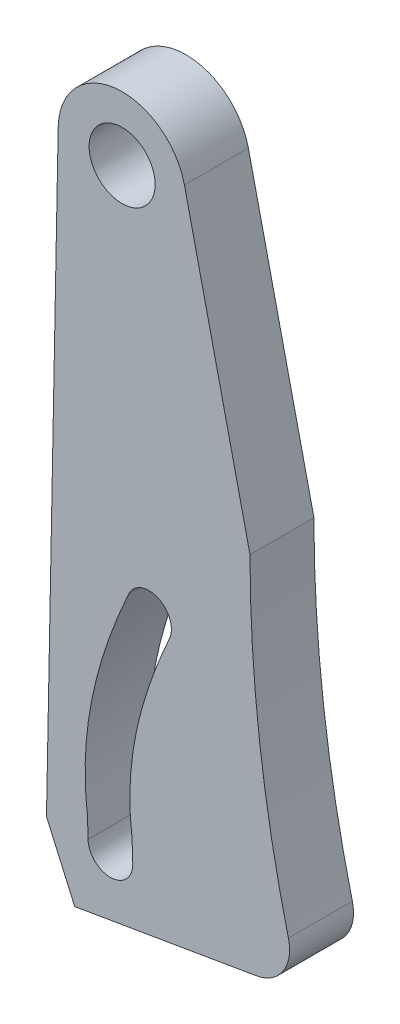
SolidWorks part; units mm, degrees
material "Thornel Mat VMA"
ref_plane "前视基准面" through (0, 0, 0) normal (0, 0, 1) x (1, 0, 0)
ref_plane "上视基准面" through (0, 0, 0) normal (0, 1, 0) x (1, 0, 0)
ref_plane "右视基准面" through (0, 0, 0) normal (1, 0, 0) x (0, 0, -1)
other "Configuration Table"
sketch "草图1"
  line L0 (3.8162, 0.7114) -> (0.7411, 14.1914)
  line L1 (-2.1838, 13.5241) -> (3.8162, -14.4209) construction
  line L2 (-2.1838, 13.5241) -> (-2.7337, -14.6313) construction
  line L3 (-2.1838, 13.5241) -> (-2.7471, -14.0898) construction
  line L4 (-2.1838, 13.5241) -> (-2.7731, -13.5291) construction
  line L5 (-2.1838, 13.5241) -> (-2.8303, -12.9865) construction
  line L6 (-2.1838, 13.5241) -> (-2.8637, -12.4261) construction
  line L7 (-2.1838, 13.5241) -> (-2.8697, -11.8608) construction
  line L8 (-2.1838, 13.5241) -> (-2.8529, -11.291) construction
  line L9 (-2.1838, 13.5241) -> (-2.8123, -10.717) construction
  line L10 (-2.1838, 13.5241) -> (-2.7482, -10.1392) construction
  line L11 (-2.1838, 13.5241) -> (-2.661, -9.5577) construction
  line L12 (-2.1838, 13.5241) -> (-2.5512, -8.9728) construction
  line L13 (-2.1838, 13.5241) -> (-2.4192, -8.3846) construction
  line L14 (-2.1838, 13.5241) -> (-2.2655, -7.793) construction
  line L15 (-2.1838, 13.5241) -> (-2.0907, -7.1983) construction
  line L16 (-2.1838, 13.5241) -> (-1.8954, -6.6001) construction
  line L17 (-2.1838, 13.5241) -> (-1.6801, -5.9985) construction
  line L18 (-2.1838, 13.5241) -> (-1.4455, -5.3931) construction
  line L19 (-2.1838, 13.5241) -> (-1.1925, -4.7837) construction
  line L20 (-2.1838, 13.5241) -> (-0.9217, -4.1699) construction
  line L21 (-0.9217, -4.1699) -> (-1.1925, -4.7837) construction
  line L22 (-1.1925, -4.7837) -> (-1.4455, -5.3931) construction
  line L23 (0.0301, -4.6131) -> (-0.9217, -4.1699) construction
  line L24 (-2.1622, -4.381) -> (-0.2228, -5.1864) construction
  line L25 (-1.4455, -5.3931) -> (-1.6801, -5.9985) construction
  line L26 (-1.6801, -5.9985) -> (-1.8954, -6.6001) construction
  line L27 (-2.4246, -5.0138) -> (-0.4664, -5.7724) construction
  line L28 (-2.6687, -5.6447) -> (-0.6915, -6.3522) construction
  line L29 (-1.8954, -6.6001) -> (-2.0907, -7.1983) construction
  line L30 (-2.8935, -6.2741) -> (-0.8972, -6.9261) construction
  line L31 (-2.0907, -7.1983) -> (-2.2655, -7.793) construction
  line L32 (-3.0981, -6.9022) -> (-1.0833, -7.4943) construction
  line L33 (-2.2655, -7.793) -> (-2.4192, -8.3846) construction
  line L34 (-3.2818, -7.529) -> (-1.2492, -8.057) construction
  line L35 (-3.4437, -8.1547) -> (-1.3946, -8.6144) construction
  line L36 (-2.4192, -8.3846) -> (-2.5512, -8.9728) construction
  line L37 (-2.5512, -8.9728) -> (-2.661, -9.5577) construction
  line L38 (-3.5831, -8.7791) -> (-1.5192, -9.1666) construction
  line L39 (-2.661, -9.5577) -> (-2.7482, -10.1392) construction
  line L40 (-3.6994, -9.402) -> (-1.6226, -9.7134) construction
  line L41 (-2.7482, -10.1392) -> (-2.8123, -10.717) construction
  line L42 (-3.7917, -10.0234) -> (-1.7046, -10.255) construction
  line L43 (-2.7482, -10.1392) -> (-2.8123, -10.717) construction
  line L44 (-2.8123, -10.717) -> (-2.8529, -11.291) construction
  line L45 (-2.8529, -11.291) -> (-2.8697, -11.8608) construction
  line L46 (-2.8697, -11.8608) -> (-2.8637, -12.4261) construction
  line L47 (-2.8637, -12.4261) -> (-2.8303, -12.9865) construction
  line L48 (-2.8303, -12.9865) -> (-2.7731, -13.5291) construction
  line L49 (-3.8597, -10.6429) -> (-1.7649, -10.7912) construction
  line L50 (-3.9025, -11.2601) -> (-1.8034, -11.3219) construction
  line L51 (-3.9196, -11.8719) -> (-1.8198, -11.8497) construction
  line L52 (-3.9119, -12.4886) -> (-1.8156, -12.3636) construction
  line L53 (-2.8303, -12.9865) -> (-2.7731, -13.5291) construction
  line L54 (-3.8745, -13.0967) -> (-1.7861, -12.8764) construction
  line L55 (-2.7731, -13.5291) -> (-2.7471, -14.0898) construction
  line L56 (-3.8219, -13.5777) -> (-1.7242, -13.4806) construction
  line L57 (-3.7968, -14.1158) -> (-1.6974, -14.0638) construction
  line L58 (-2.7471, -14.0898) -> (-2.7337, -14.6313) construction
  line L59 (-2.7337, -14.6313) -> (-1.684, -14.6053) construction
  line L60 (-2.7337, -14.6313) -> (-3.7834, -14.6573) construction
  line L61 (-2.7337, -14.6313) -> (-4.4081, -17.7048) construction
  line L62 (-2.7337, -14.6313) -> (-5.7328, -14.7056) construction
  line L63 (-4.4081, -17.7048) -> (4.1278, -16.2526)
  line L64 (-5.7328, -14.7056) -> (-4.4081, -17.7048)
  line L65 (-5.7328, -14.7056) -> (-5.1832, 13.5824)
  line L66 (-0.9217, -4.1699) -> (-1.8824, -3.7461) construction
  circle A0 centre (-2.1838, 13.5241) radius 1.55
  arc A1 (3.8162, 0.7114) -> (5.619, -13.9714) centre (64.5084, 0.7114) ccw
  arc A2 (0.7411, 14.1914) -> (-5.1832, 13.5824) centre (-2.1838, 13.5241) ccw
  arc A3 (4.1278, -16.2526) -> (5.619, -13.9714) centre (3.8162, -14.4209) ccw
  arc A4 (-3.7834, -14.6573) -> (-1.684, -14.6053) centre (-2.7337, -14.6313) ccw
  arc A12 (0.0301, -4.6131) -> (-1.8824, -3.7461) centre (-0.9217, -4.1699) ccw
  spline S0 degree 3 poles (-3.7834, -14.6573) (-3.7993, -14.2982) (-3.7863, -13.7741) (-3.8865, -13.0558) (-3.9159, -12.4861) (-3.9238, -11.8735) (-3.9066, -11.2577) (-3.8491, -10.4322) (-3.741, -9.6037) (-3.5864, -8.7763) (-3.4467, -8.1517) (-3.2845, -7.5259) (-3.1005, -6.8989) (-2.8956, -6.2707) (-2.6705, -5.6411) (-2.3426, -4.7944) (-2.072, -4.1648) (-1.8824, -3.7461) knots 0 0 0 0 0.09621 0.139298 0.193554 0.248477 0.302979 0.358078 0.469497 0.525932 0.582904 0.640455 0.698625 0.757451 0.81697 0.877215 1 1 1 1
  spline S1 degree 3 poles (-1.684, -14.6053) (-1.6984, -14.2309) (-1.6906, -13.6511) (-1.7908, -12.9082) (-1.8196, -12.3636) (-1.8228, -11.845) (-1.8071, -11.3204) (-1.7682, -10.7884) (-1.7076, -10.2519) (-1.6254, -9.71) (-1.486, -8.9741) (-1.3512, -8.4238) (-1.2492, -8.057) knots 0 0 0 0 0.170355 0.262297 0.340044 0.417824 0.497759 0.578301 0.659977 0.742887 0.827132 1 1 1 1
  spline S2 degree 3 poles (0.0301, -4.6131) (-0.1433, -4.9961) (-0.3915, -5.5728) (-0.6925, -6.3475) (-0.9647, -7.1056) (-1.1434, -7.6766) (-1.2492, -8.057) knots 0 0 0 0 0.34298 0.512099 0.67788 1 1 1 1
other "对齐组1" parameters "D1"=3.1, "D2"=3.1, "D3"=6, "D4"=3.1, "D6"=60.6922, "D9"=3.716, "D29"=1.6132, "D31"=2, "D33"=2, "D35"=2, "D37"=2, "D39"=2, "D41"=2, "D43"=2, "D45"=2, "D47"=2, "D49"=2, "D52"=10.768, "D59"=2.05, "D71"=2, "D84"=2, "D85"=2.1, "D5"=13.8263, "D7"=3.8162, "D8"=5.619, "D10"=3.8162, "D11"=26.7925, "D12"=26.7823, "D13"=26.7925, "D14"=25.5532, "D15"=26.2854, "D16"=27.0533, "D17"=21.6117, "D18"=19.2403, "D19"=20.3681, "D20"=20.7218, "D21"=22.5274, "D22"=24.4408, "D23"=20.4903, "D24"=21.1433, "D25"=20.0275, "D26"=17.4108, "D27"=21.8201, "D28"=20.5543, "D30"=27.945, "D32"=16.1585, "D34"=21.91, "D36"=21.3173, "D38"=18.0374, "D40"=15.8792, "D42"=15.2189, "D44"=14.1906, "D46"=18.3346, "D48"=17.739, "D50"=1, "D51"=0.6492, "D53"=1, "D54"=1, "D55"=0.8492, "D56"=0.8492, "D57"=0.6292, "D58"=1.1033, "D60"=1.1166, "D61"=0.6111, "D62"=1.142, "D63"=1.3101, "D64"=0.6029, "D65"=0.5951, "D66"=1.0637, "D67"=0.588, "D68"=1.2009, "D69"=0.5814, "D70"=1.0157, "D72"=0.5754, "D73"=0.402, "D74"=0.402, "D75"=1.1507, "D76"=1.1506, "D77"=0.9199, "D78"=0.9199, "D79"=0.5456, "D80"=0.8413, "D81"=0.5613, "D82"=1.1715, "D83"=1.1711, "D86"=8.6586
other "对齐组2"
extrude "凸台-拉伸1" add sketch "草图1" along normal blind 3
